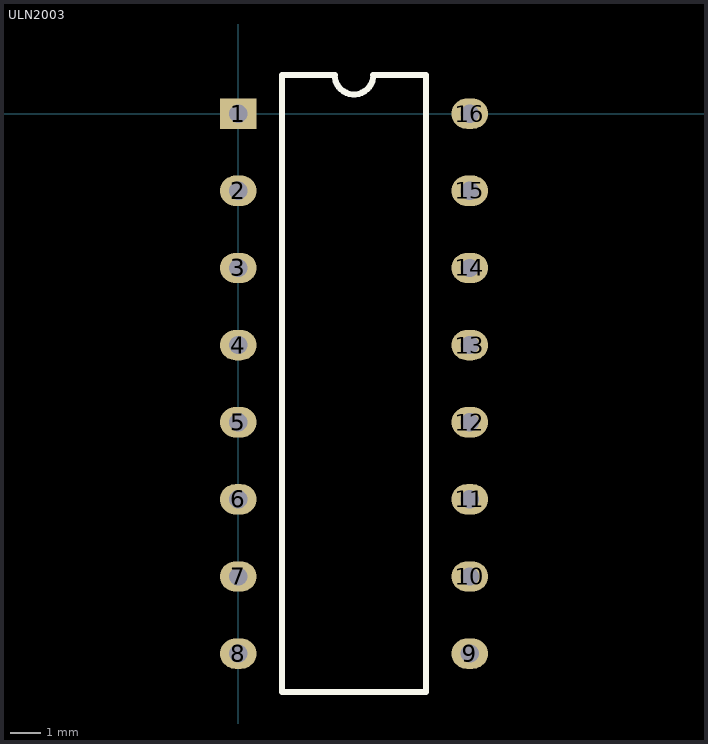
[diagram p0: the footprints below, top view; thin cyan lines are the x and y axes]
# Altium footprint library MISC86340-15.PcbLib: 2 footprints
Each footprint in its own frame and in the unit in brackets; x right, y up, seen from the top. Pads: shape width x height; smd on the part's side, far side on the other; paste and mask are expansions set on the pad; w line width, h text height; cw(c..) or ccw(c..) is an arc to the next point about the centre after c.

## LC-DIP-16 [mm]

## ULN2003 [mm]
pads (16):
  rect 1.2x1 hole 0.6: 1(0,0)
  oval 1.2x1 hole 0.6: 2(0,-2.54) 3(0,-5.08) 4(0,-7.62) 5(0,-10.16) 6(0,-12.7) 7(0,-15.24) 8(0,-17.78) 9(7.62,-17.78) 10(7.62,-15.24) 11(7.62,-12.7) 12(7.62,-10.16) 13(7.62,-7.62) 14(7.62,-5.08) 15(7.62,-2.54) 16(7.62,0)
Top Overlay:
  lines w0.2: 1.435,-19.05 6.185,-19.05 6.185,1.27 4.445,1.27 cw(c3.81,1.27) 3.175,1.27 1.435,1.27 1.435,-19.05